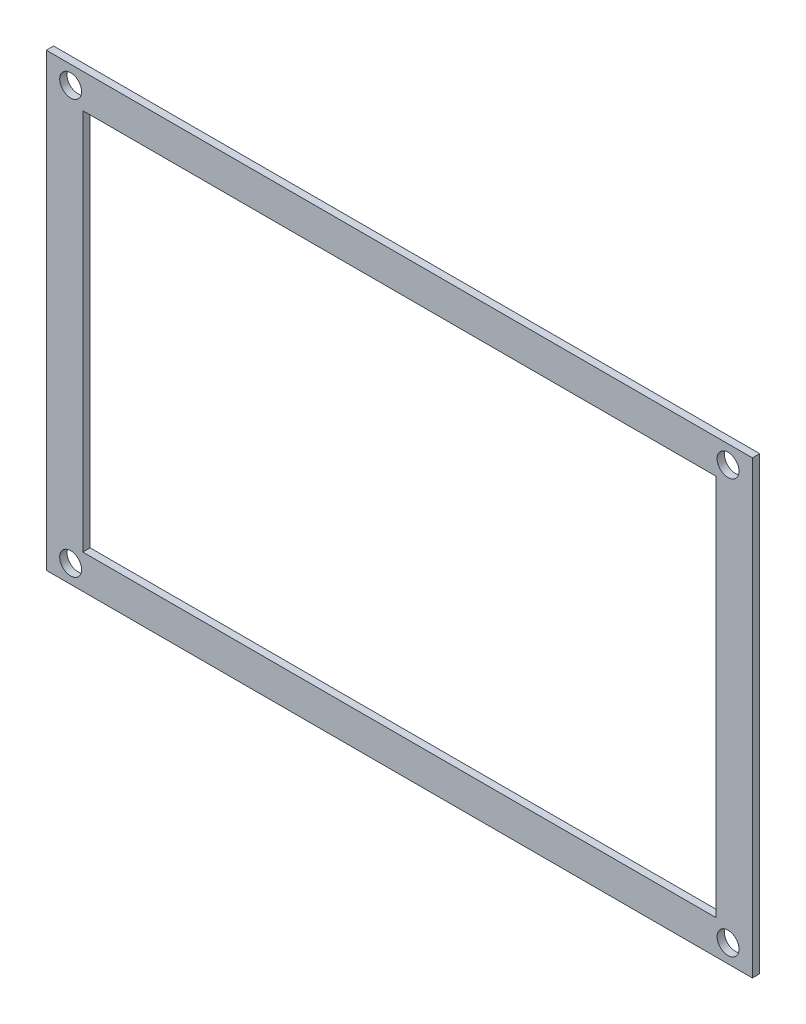
SolidWorks part; units mm, degrees
material "Plain Carbon Steel"
ref_plane "Front Plane" through (0, 0, 0) normal (0, 0, 1) x (1, 0, 0)
ref_plane "Top Plane" through (0, 0, 0) normal (0, 1, 0) x (1, 0, 0)
ref_plane "Right Plane" through (0, 0, 0) normal (1, 0, 0) x (0, 0, -1)
sketch "Sketch1" plane through (0, 0, 0) normal (0, 0, 1) x (1, 0, 0)
  line L0 (0, -2945.5618) -> (0, 144332.527) construction
  line L1 (-2945.5618, 0) -> (144332.527, 0) construction
  line L3 (-145, 92.5) -> (145, 92.5)
  line L4 (-145, 92.5) -> (-145, -92.5)
  line L5 (-145, -92.5) -> (145, -92.5)
  line L6 (145, 92.5) -> (145, -92.5)
  line L7 (-130, 78.5) -> (130, 78.5)
  line L8 (-130, 78.5) -> (-130, -78.5)
  line L9 (-130, -78.5) -> (130, -78.5)
  line L10 (130, 78.5) -> (130, -78.5)
  dimension "D1" = 185
  dimension "D2" = 290
  dimension "D3" = 260
  dimension "D4" = 157
extrude "Boss-Extrude1" add sketch "Sketch1" along normal blind 3
sketch "Sketch2" plane through (0, 0, 3) normal (0, 0, 1) x (1, 0, 0)
  circle A0 centre (-135, 85) radius 4.5
  dimension "D3" = 9
  dimension "D1" = 135
  dimension "D2" = 85
extrude "Cut-Extrude1" cut sketch "Sketch2" against normal blind 3
pattern_linear "LPattern1" count 2 spacing 270 along (1, 0, 0) count 2 spacing 170 along (0, -1, 0) of "Cut-Extrude1"
